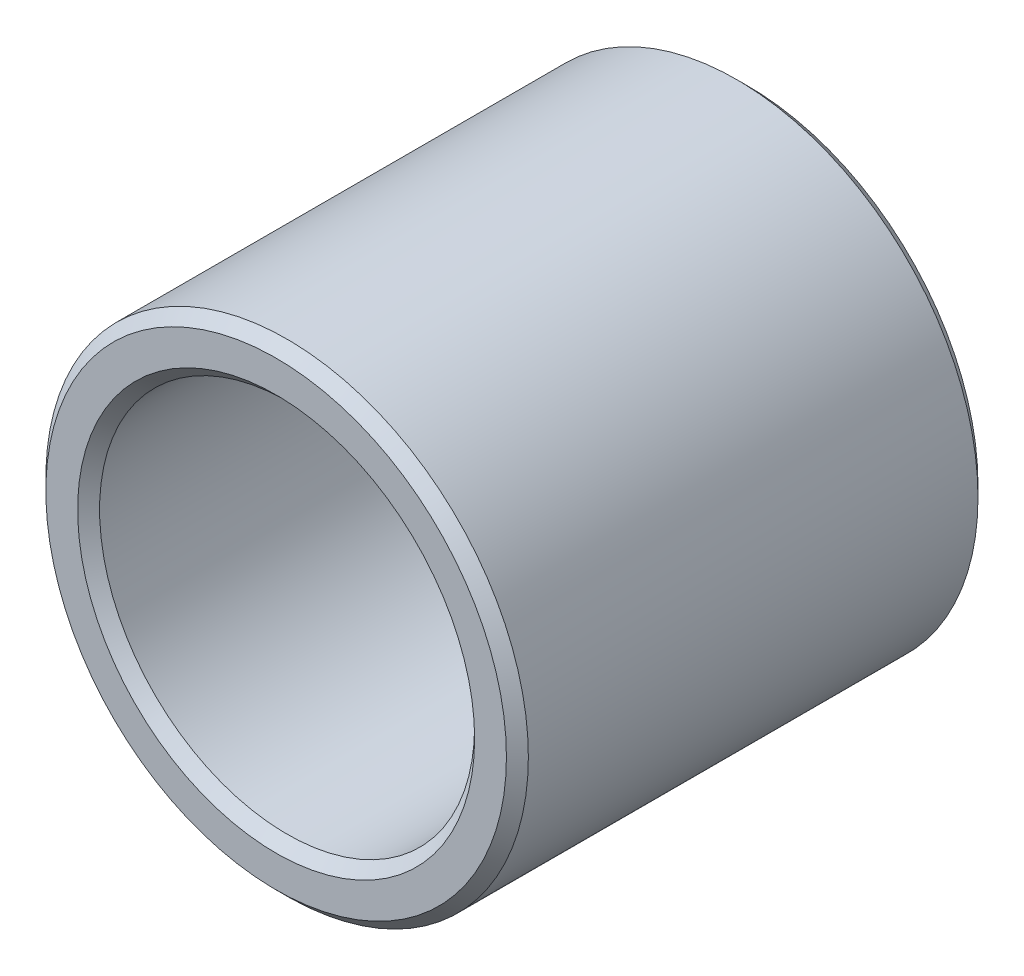
from build123d import *

# Parameters (mm, degrees)
SKETCH_1_R      = 11
SKETCH_1_R_2    = 8.55
EXTRUDE_1_DEPTH = 21.5
CHAMFER_1_SIZE  = 0.5


with BuildPart() as part:
    # 草图1 → 凸台-拉伸1 (new body)
    with BuildSketch(Plane.XY):
        Circle(SKETCH_1_R)
        Circle(SKETCH_1_R_2, mode=Mode.SUBTRACT)
    extrude(amount=EXTRUDE_1_DEPTH)

    # 倒角1
    chamfer_1_edges = [part.edges().sort_by_distance(p)[0] for p in [
        (-11, 0, 0),
        (-11, 0, 21.5),
        (-8.55, 0, 0),
        (-8.55, 0, 21.5),
    ]]
    chamfer(chamfer_1_edges, length=CHAMFER_1_SIZE)


solid = part.part
